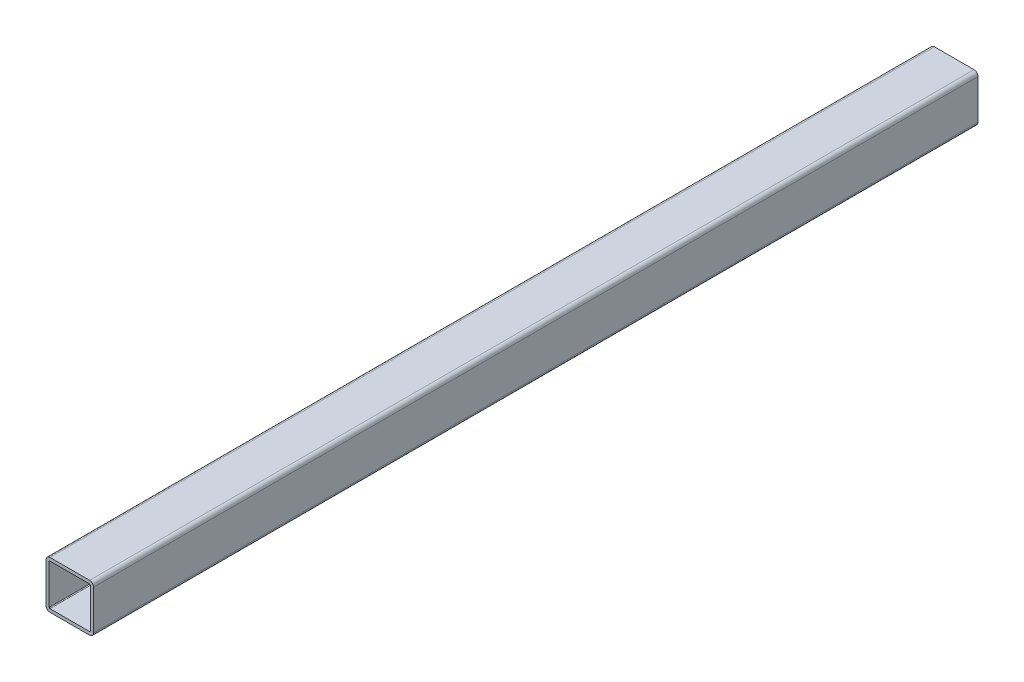
from build123d import *

# Parameters (mm, degrees)
SKETCH1_W           = 60
SKETCH1_H           = 60
BOSS_EXTRUDE1_DEPTH = 1116
FILLET1_R           = 5
SHELL1_T            = -4


with BuildPart() as part:
    # Sketch1 → Boss-Extrude1 (new body)
    with BuildSketch(Plane.XY):
        Rectangle(SKETCH1_W, SKETCH1_H)
    extrude(amount=BOSS_EXTRUDE1_DEPTH)

    # Fillet1
    fillet1_edges = [part.edges().sort_by_distance(p)[0] for p in [
        (30, -30, 558),
        (30, 30, 558),
        (-30, 30, 558),
        (-30, -30, 558),
    ]]
    fillet(fillet1_edges, radius=FILLET1_R)

    # Shell1
    shell1_openings = [part.faces().sort_by_distance(p)[0] for p in [
        (0, 0, 1116),
        (0, 0, 0),
    ]]
    offset(amount=SHELL1_T, openings=shell1_openings, kind=Kind.INTERSECTION)


solid = part.part
